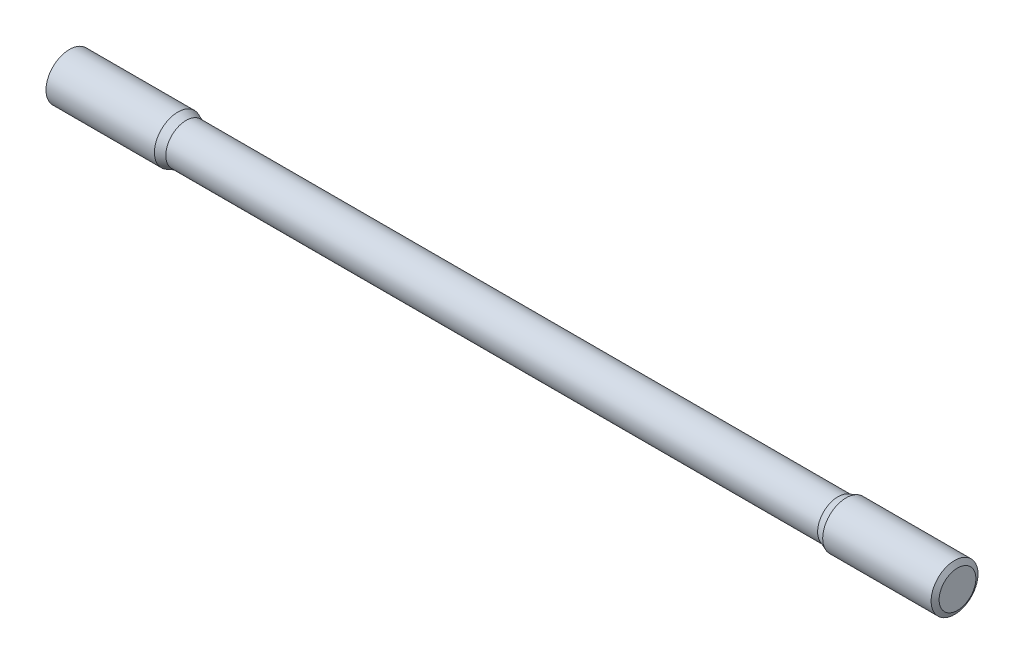
SolidWorks part; units mm, degrees
ref_plane "前视" through (0, 0, 0) normal (0, 0, 1) x (1, 0, 0)
ref_plane "上视" through (0, 0, 0) normal (0, 1, 0) x (1, 0, 0)
ref_plane "右视" through (0, 0, 0) normal (1, 0, 0) x (0, 0, -1)
sketch "尺寸草图" plane through (0, 0, 0) normal (0, 0, 1) x (1, 0, 0)
  line L0 (0, 0) -> (2, 0) construction
  line L1 (2, 0) -> (4, 0) construction
  line L2 (-263.6, 0) -> (16.4, 0) construction
  point P3 (16, 0)
  point P4 (38, 0)
  point P5 (2.8, 0)
  point P6 (2, 0)
  point P7 (16.4, 0)
  point P8 (2, 0)
  point P9 (4, 0)
  point P10 (-263.6, 0)
  dimension "D1" = 2
  dimension "l" = 280
  dimension "d" = 16
  dimension "b" = 38
  dimension "X" = 2.8
  dimension "ds" = 14.4
  dimension "P" = 2
sketch "草图1" plane through (0, 0, 0) normal (0, 0, 1) x (1, 0, 0)
  line L0 (-152, 0) -> (212.3418, 0) construction
  line L1 (-152, 8) -> (-114, 8)
  line L2 (-111.2, 6.928) -> (111.2, 6.928)
  line L3 (-152, 8) -> (-152, 0)
  line L4 (0, 0) -> (0, -10.5843) construction
  line L5 (-114, 8) -> (-111.2, 6.928)
  line L6 (152, 0) -> (-152, 0)
  line L7 (114, 8) -> (111.2, 6.928)
  line L8 (152, 8) -> (152, 0)
  line L9 (152, 8) -> (114, 8)
  point P13 (0, 6.928)
  dimension "X" = 2.8
  dimension "l/2" = 152
  dimension "b" = 38
  dimension "d/2" = 8
  dimension "中径" = 6.928
revolve "基体-旋转" add sketch "草图1"
cosmetic thread "装饰螺纹线1"
revolve "螺纹切除" cut sketch "草图2" angle 360 about L5
sketch "草图2" plane through (0, 0, 0) normal (0, 0, 1) x (1, 0, 0)
  line L0 (-153, 8) -> (-151, 8)
  line L1 (-151, 8) -> (-152, 6.268)
  line L2 (-152, 6.268) -> (-153, 8)
  line L3 (-114, 8) -> (-152, 8) construction
  line L4 (-152, 8) -> (-152, -8) construction
  line L5 (-26.9524, 0) -> (-19.4497, 0) construction
  line L6 (-152, 0) -> (212.3418, 0) construction
  dimension "D1" = 60
  dimension "D2" = 60
  dimension "D3" = 1.732
pattern_linear "左螺纹阵列" [suppressed] count 20 spacing 2
cosmetic thread "装饰螺纹线2"
mirror "镜向1" about plane through (0, 0, 0) normal (1, 0, 0) of "螺纹切除"
mirror "镜向2" [suppressed] about plane through (0, 0, 0) normal (1, 0, 0)
